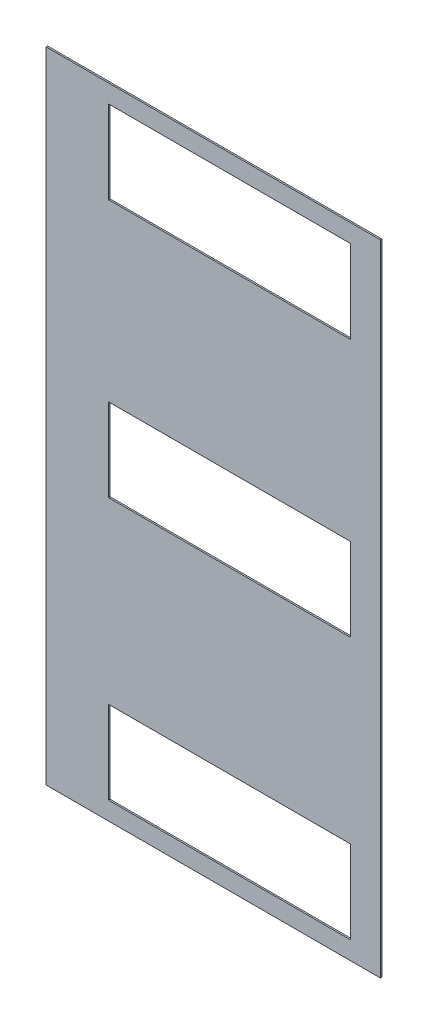
SolidWorks part; units mm, degrees
ref_plane "Front Plane" through (0, 0, 0) normal (0, 0, 1) x (1, 0, 0)
ref_plane "Top Plane" through (0, 0, 0) normal (0, 1, 0) x (1, 0, 0)
ref_plane "Right Plane" through (0, 0, 0) normal (1, 0, 0) x (0, 0, -1)
other "Configuration Table"
sketch "Sketch1" plane through (0, 0, 0) normal (0, 0, 1) x (1, 0, 0)
  line L0 (0, 2124) -> (1110.6118, 2124)
  line L1 (1110.6118, 2124) -> (1110.6118, 0)
  line L2 (1110.6118, 0) -> (0, 0)
  line L3 (0, 0) -> (0, 2124)
  line L4 (207.0516, 2063.6568) -> (1012.0741, 2063.6568)
  line L5 (1012.0741, 2063.6568) -> (1012.0741, 1787.8953)
  line L6 (1012.0741, 1787.8953) -> (207.0516, 1787.8953)
  line L7 (207.0516, 1787.8953) -> (207.0516, 2063.6568)
  line L8 (207.0516, 1206.4398) -> (1012.0741, 1206.4398)
  line L9 (1012.0741, 1206.4398) -> (1012.0741, 930.6782)
  line L10 (1012.0741, 930.6782) -> (207.0516, 930.6782)
  line L11 (207.0516, 930.6782) -> (207.0516, 1206.4398)
  line L12 (207.0516, 336.0126) -> (1012.0741, 336.0126)
  line L13 (1012.0741, 336.0126) -> (1012.0741, 60.251)
  line L14 (1012.0741, 60.251) -> (207.0516, 60.251)
  line L15 (207.0516, 60.251) -> (207.0516, 336.0126)
  dimension "D1" = 207.0516
  dimension "D2" = 1012.0741
  dimension "D3" = 1110.6118
  dimension "D4" = 60.251
  dimension "D5" = 336.0126
  dimension "D6" = 930.6782
  dimension "D7" = 1787.8953
  dimension "D8" = 2124
extrude "Boss-Extrude1" add sketch "Sketch1" along normal blind 5
